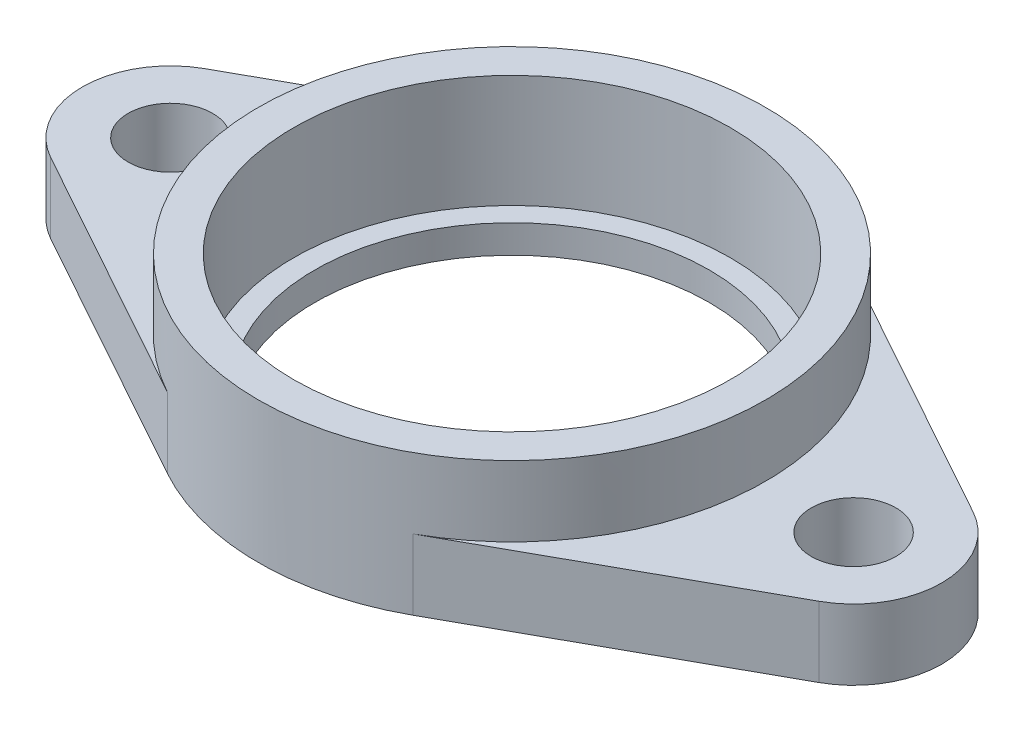
SolidWorks part; units mm, degrees
ref_plane "前视基准面" through (0, 0, 0) normal (0, 0, 1) x (1, 0, 0)
ref_plane "上视基准面" through (0, 0, 0) normal (0, 1, 0) x (1, 0, 0)
ref_plane "右视基准面" through (0, 0, 0) normal (1, 0, 0) x (0, 0, -1)
sketch "草图1" plane through (0, 0, 0) normal (0, 1, 0) x (1, 0, 0)
  line L0 (-54.5567, 10.9346) -> (-17.4433, 31.4918)
  line L1 (17.4433, 31.4918) -> (54.5567, 10.9346)
  line L2 (54.5567, -10.9346) -> (17.4433, -31.4918)
  line L3 (-17.4433, -31.4918) -> (-54.5567, -10.9346)
  arc A0 (-17.4433, -31.4918) -> (17.4433, -31.4918) centre (0, 0) ccw
  arc A1 (54.5567, -10.9346) -> (54.5567, 10.9346) centre (48.5, 0) ccw
  circle A2 centre (48.5, 0) radius 6
  arc A3 (-54.5567, 10.9346) -> (-54.5567, -10.9346) centre (-48.5, 0) ccw
  circle A4 centre (-48.5, 0) radius 6
  arc A5 (17.4433, 31.4918) -> (-17.4433, 31.4918) centre (0, 0) ccw
  dimension "D1" = 48.5
  dimension "D2" = 48.5
extrude "凸台-拉伸1" add sketch "草图1" along normal blind 10
sketch "草图2" plane through (0, 10, 0) normal (0, 1, 0) x (1, 0, 0)
  circle A0 centre (0, 0) radius 36
extrude "凸台-拉伸2" add sketch "草图2" along normal blind 10
sketch "草图3" plane through (0, 20, 0) normal (0, 1, 0) x (1, 0, 0)
  circle A0 centre (0, 0) radius 31
extrude "切除-拉伸1" cut sketch "草图3" against normal blind 16
sketch "草图4" plane through (0, 4, 0) normal (0, 1, 0) x (1, 0, 0)
  circle A0 centre (0, 0) radius 28
extrude "切除-拉伸2" cut sketch "草图4" against normal blind 16
